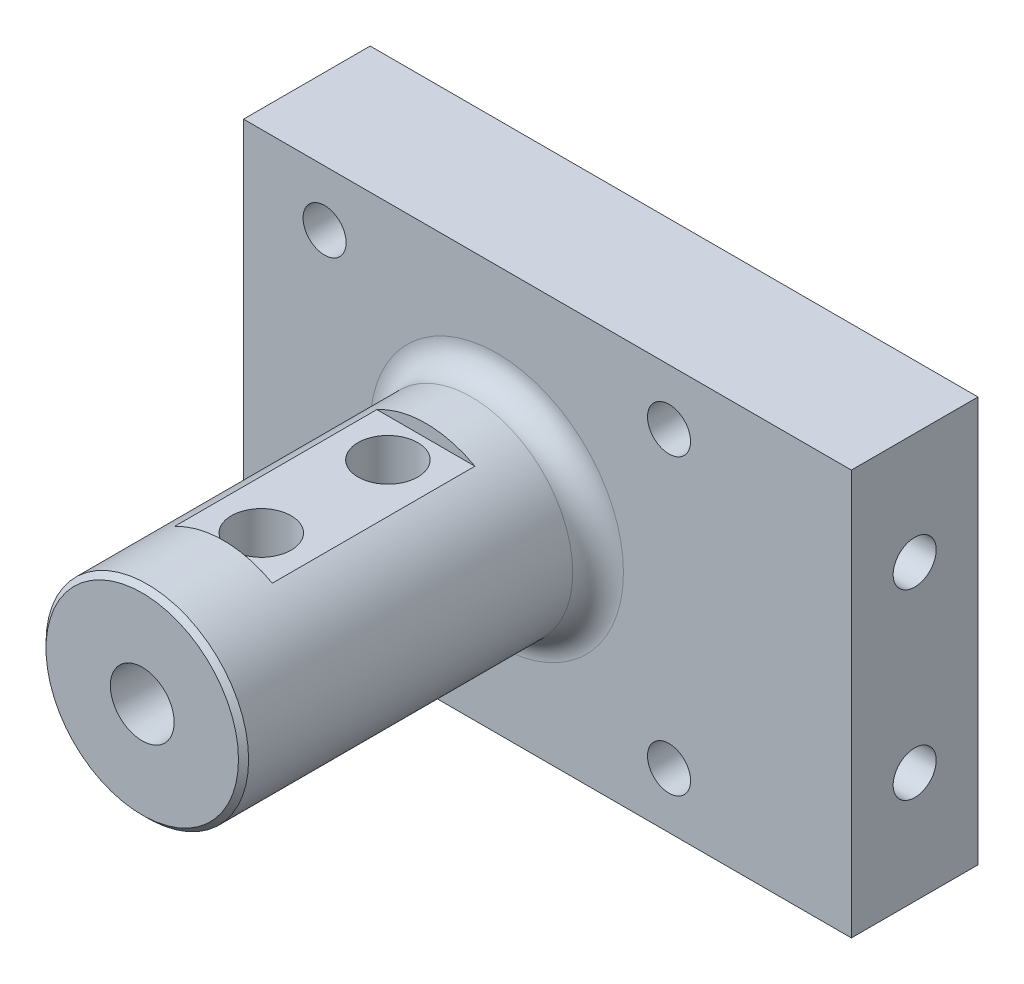
from build123d import *

# Parameters (mm, degrees)
SKETCH_13_W                 = 100
SKETCH_13_H                 = 80
EXTRUDE_3_DEPTH             = 25
SKETCH_14_R                 = 0.5
CUT_EXTRUDE_4_DEPTH         = 18
SKETCH_15_R                 = 20
EXTRUDE_4_DEPTH             = 70
HOLE_WIZARD_10_0_10_1_D     = 10
HOLE_WIZARD_10_0_10_1_DEPTH = 25
HOLE_WIZARD_10_0_10_1_TIP   = 3.004303095
SKETCH_21_OUTSIDE_W         = 133.89
SKETCH_21_OUTSIDE_H         = 113.89
SKETCH_21_OUTSIDE_W_2       = 54.577135948
SKETCH_21_OUTSIDE_H_2       = 35
CUT_EXTRUDE_5_DEPTH         = 40
HOLE_WIZARD_G1_4_1_D        = 11.8
HOLE_WIZARD_G1_4_1_DEPTH    = 25
HOLE_WIZARD_G1_4_1_TIP      = 3.545077652
CHAMFER_1_SIZE              = 1
HOLE_WIZARD_M10_1_D         = 8.5
HOLE_WIZARD_M10_1_DEPTH     = 27.5
HOLE_WIZARD_M10_1_TIP       = 2.553657631
FILLET_1_R                  = 5
HOLE_WIZARD_M6_1_D          = 5
HOLE_WIZARD_M6_1_DEPTH      = 35
HOLE_WIZARD_M6_1_TIP        = 1.502151548
SKETCH_35_W                 = 25
SKETCH_35_H                 = 80
EXTRUDE_7_DEPTH             = 20
HOLE_WIZARD_M10_4_D         = 8.5
HOLE_WIZARD_M10_4_DEPTH     = 27.5
HOLE_WIZARD_M10_4_TIP       = 2.553657631


with BuildPart() as part:
    # 草图13 → 凸台-拉伸3 (new body)
    with BuildSketch(Plane.XY):
        Rectangle(SKETCH_13_W, SKETCH_13_H)
    extrude(amount=EXTRUDE_3_DEPTH)

    # 草图14 → 切除-拉伸4 (cut)
    with BuildSketch(Plane.XY.offset(25)):
        with Locations((-34, 29)):
            Circle(SKETCH_14_R)
        with Locations((34, 29)):
            Circle(SKETCH_14_R)
        with Locations((34, -29)):
            Circle(SKETCH_14_R)
        with Locations((-34, -29)):
            Circle(SKETCH_14_R)
    extrude(amount=-CUT_EXTRUDE_4_DEPTH, mode=Mode.SUBTRACT)

    # 草图15 → 凸台-拉伸4 (add)
    with BuildSketch(Plane.XY.offset(25)):
        with Locations(Location((0, 0, 0), (0, 0, 180))):
            Circle(SKETCH_15_R)
    extrude(amount=EXTRUDE_4_DEPTH)

    # Ø10.0 (10) 直径孔1
    with Locations(Plane.XY.offset(95)):
        with Locations((0, 0)):
            Hole(HOLE_WIZARD_10_0_10_1_D / 2, depth=HOLE_WIZARD_10_0_10_1_DEPTH)
            with Locations((0, 0, -(HOLE_WIZARD_10_0_10_1_DEPTH + HOLE_WIZARD_10_0_10_1_TIP / 2))):  # 118° drill point
                Cone(0, HOLE_WIZARD_10_0_10_1_D / 2, HOLE_WIZARD_10_0_10_1_TIP, mode=Mode.SUBTRACT)

    # 草图19 → 切除-旋转10 (revolve, cut)
    with BuildSketch(Plane(origin=(0, 0, 0), x_dir=(1, 0, 0), z_dir=(0, 1, 0)), mode=Mode.PRIVATE) as cut_revolve_10_sk:
        Polygon((-6.3, -95), (-5.65, -82), (-5, -82), (-5, -95), align=None)
    revolve(cut_revolve_10_sk.sketch.rotate(Axis((0, 0, 95), (0, 0, -1)), 180), axis=Axis((0, 0, 95), (0, 0, -1)), mode=Mode.SUBTRACT)

    # 草图21 outside → 切除-拉伸5 (cut)
    with BuildSketch(Plane.XY.offset(79)):
        Rectangle(SKETCH_21_OUTSIDE_W, SKETCH_21_OUTSIDE_H)
        Rectangle(SKETCH_21_OUTSIDE_W_2, SKETCH_21_OUTSIDE_H_2, mode=Mode.SUBTRACT)
    extrude(amount=-CUT_EXTRUDE_5_DEPTH, mode=Mode.SUBTRACT)

    # G1/4 螺纹孔1
    with Locations(Plane(origin=(0, 17.5, 0), x_dir=(1, 0, 0), z_dir=(0, 1, 0))):
        with Locations((0, -71.5), (0, -46.5)):
            Hole(HOLE_WIZARD_G1_4_1_D / 2, depth=HOLE_WIZARD_G1_4_1_DEPTH)
            with Locations((0, 0, -(HOLE_WIZARD_G1_4_1_DEPTH + HOLE_WIZARD_G1_4_1_TIP / 2))):  # 118° drill point
                Cone(0, HOLE_WIZARD_G1_4_1_D / 2, HOLE_WIZARD_G1_4_1_TIP, mode=Mode.SUBTRACT)

    # 倒角1
    chamfer_1_edges = [part.edges().sort_by_distance(p)[0] for p in [
        (20, 0, 95),
    ]]
    chamfer(chamfer_1_edges, length=CHAMFER_1_SIZE)

    # M10 螺纹孔1
    with Locations(Plane.XY.offset(25)):
        with Locations((-34, 29), (34, 29), (34, -29), (-34, -29)):
            Hole(HOLE_WIZARD_M10_1_D / 2, depth=HOLE_WIZARD_M10_1_DEPTH)
            with Locations((0, 0, -(HOLE_WIZARD_M10_1_DEPTH + HOLE_WIZARD_M10_1_TIP / 2))):  # 118° drill point
                Cone(0, HOLE_WIZARD_M10_1_D / 2, HOLE_WIZARD_M10_1_TIP, mode=Mode.SUBTRACT)

    # 圆角1
    fillet_1_edges = [part.edges().sort_by_distance(p)[0] for p in [
        (20, 0, 25),
    ]]
    fillet(fillet_1_edges, radius=FILLET_1_R)

    # M6 螺纹孔1
    with Locations(Plane.XY.offset(69)):
        with Locations((0, 0)):
            Hole(HOLE_WIZARD_M6_1_D / 2, depth=HOLE_WIZARD_M6_1_DEPTH)
            with Locations((0, 0, -(HOLE_WIZARD_M6_1_DEPTH + HOLE_WIZARD_M6_1_TIP / 2))):  # 118° drill point
                Cone(0, HOLE_WIZARD_M6_1_D / 2, HOLE_WIZARD_M6_1_TIP, mode=Mode.SUBTRACT)

    # 草图35 → 凸台-拉伸7 (add)
    with BuildSketch(Plane(origin=(50, 0, 0), x_dir=(0, 0, -1), z_dir=(1, 0, 0))):
        with Locations((-12.5, 0)):
            Rectangle(SKETCH_35_W, SKETCH_35_H)
    extrude(amount=EXTRUDE_7_DEPTH)

    # M10 螺纹孔4
    with Locations(Plane(origin=(70, 0, 0), x_dir=(0, 0, -1), z_dir=(1, 0, 0))):
        with Locations((-12.5, 18), (-12.5, -18)):
            Hole(HOLE_WIZARD_M10_4_D / 2, depth=HOLE_WIZARD_M10_4_DEPTH)
            with Locations((0, 0, -(HOLE_WIZARD_M10_4_DEPTH + HOLE_WIZARD_M10_4_TIP / 2))):  # 118° drill point
                Cone(0, HOLE_WIZARD_M10_4_D / 2, HOLE_WIZARD_M10_4_TIP, mode=Mode.SUBTRACT)


solid = part.part
